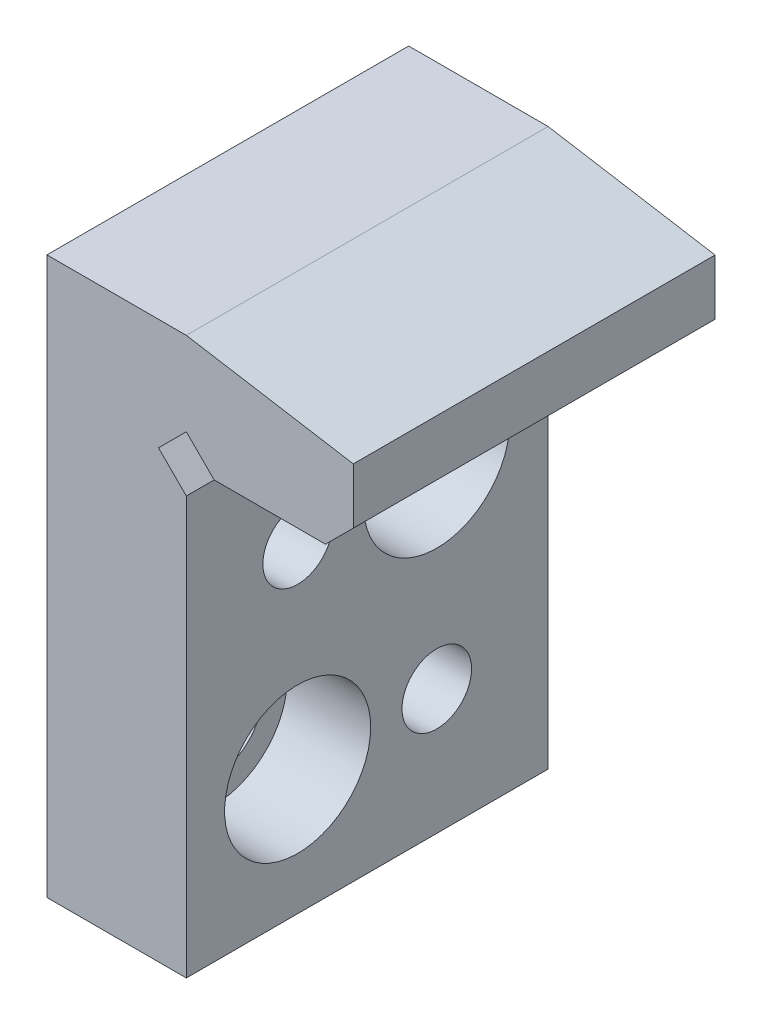
SolidWorks part; units mm, degrees
material "S45C"
ref_plane "Front Plane" through (0, 0, 0) normal (0, 0, 1) x (1, 0, 0)
ref_plane "Top Plane" through (0, 0, 0) normal (0, 1, 0) x (1, 0, 0)
ref_plane "Right Plane" through (0, 0, 0) normal (1, 0, 0) x (0, 0, -1)
sketch "Sketch1" plane through (0, 0, 0) normal (0, 0, 1) x (1, 0, 0)
  line L0 (55.1681, 40.7066) -> (57.1681, 42.7066)
  line L1 (47.1681, 40.7066) -> (55.1681, 40.7066)
  line L2 (45.1681, 48.7066) -> (35.1503, 48.7066)
  line L3 (45.1681, 42.7066) -> (47.1681, 40.7066)
  line L4 (45.1681, 8.7066) -> (45.1681, 38.7066)
  line L5 (57.1681, 42.7066) -> (57.1681, 46.7066)
  line L6 (45.1681, 38.7066) -> (43.1681, 40.7066)
  line L7 (43.1681, 40.7066) -> (45.1681, 42.7066)
  line L8 (35.1503, 8.7066) -> (45.1681, 8.7066)
  line L9 (35.1503, 14.7066) -> (35.1503, 48.7066)
  line L10 (35.1503, 8.7066) -> (35.1503, 14.7066)
  line L11 (57.1681, 46.7066) -> (45.1681, 48.7066)
extrude "Boss-Extrude1" add sketch "Sketch1" along normal mid plane 26
sketch "Sketch2" plane through (45.1681, 0, 0) normal (1, 0, 0) x (0, 0, -1)
  line L0 (-5, 0) -> (-5, 54.2003) construction
  line L1 (5, 5.6169) -> (5, 54.9015) construction
  line L2 (-13, 8.7066) -> (-13, 38.7066) construction
  line L3 (-28.1283, 17.7066) -> (30.0035, 17.7066) construction
  line L4 (-25.8203, 31.7066) -> (32.8885, 31.7066) construction
  line L5 (-13, 8.7066) -> (13, 8.7066) construction
  circle A0 centre (-5, 17.7066) radius 3.5
  circle A1 centre (5, 31.7066) radius 3.5
  circle A2 centre (5, 17.7066) radius 2.5
  circle A3 centre (-5, 31.7066) radius 2.5
  dimension "D5" = 5
  dimension "D6" = 7
  dimension "D1" = 8
  dimension "D2" = 10
  dimension "D3" = 9
  dimension "D4" = 14
extrude "Cut-Extrude1" cut sketch "Sketch2" against normal blind 26
sketch "Sketch3" plane through (45.1681, 0, 0) normal (1, 0, 0) x (0, 0, -1)
  circle A0 centre (5, 31.7066) radius 5.25
  circle A1 centre (-5, 17.7066) radius 5.25
  dimension "D1" = 10.5
extrude "Cut-Extrude2" cut sketch "Sketch3" against normal blind 6
